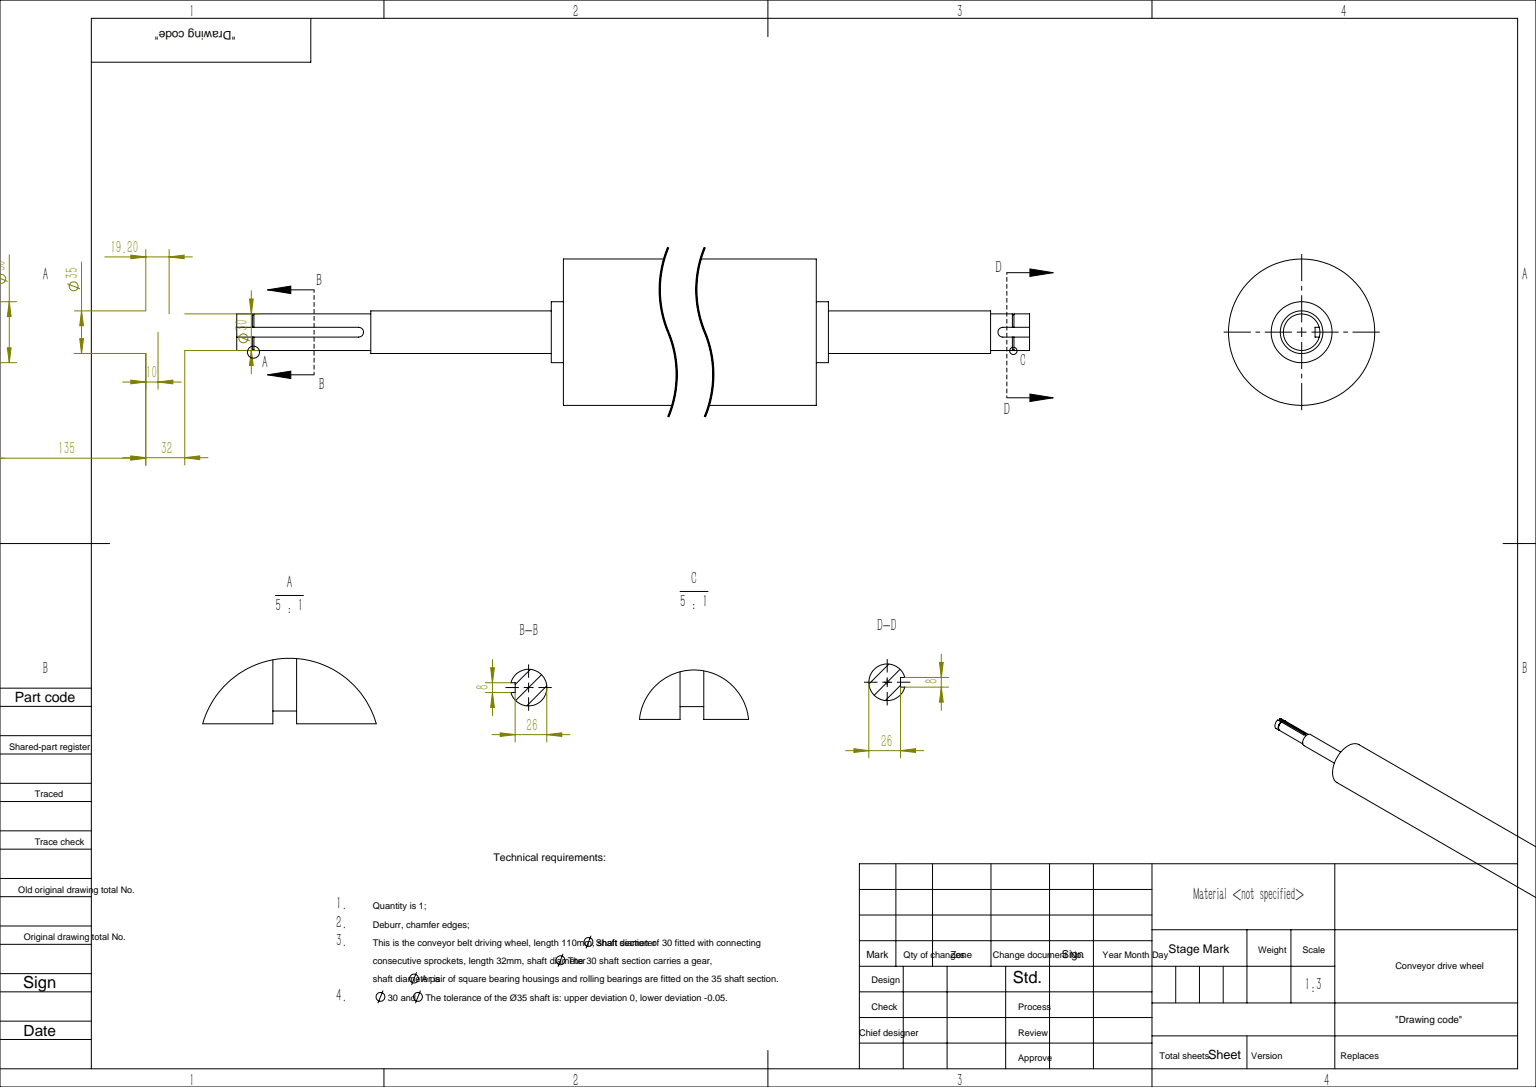
from build123d import *

# Parameters (mm, degrees)
CUT_EXTRUDE_1_DEPTH = 4
CUT_EXTRUDE_START   = -1.3
SKETCH_3_R          = 15
SKETCH_3_R_2        = 14.3
CUT_EXTRUDE_2_DEPTH = 1.3
CUT_EXTRUDE_3_DEPTH = 4
SKETCH_5_R          = 15
SKETCH_5_R_2        = 14.3
CUT_EXTRUDE_4_DEPTH = 1.3


with BuildPart() as part:
    # 草图1 → 旋转1 (revolve)
    with BuildSketch(Plane.XY, mode=Mode.PRIVATE) as revolve_1_sk:
        Polygon((0, 0), (0, 15), (110, 15), (110, 17.5), (258, 17.5), (258, 25), (268, 25), (268, 60), (1118, 60), (1118, 25), (1128, 25), (1128, 17.5), (1261, 17.5), (1261, 15), (1293, 15), (1293, 0), align=None)
    revolve(revolve_1_sk.sketch.rotate(Axis((0, 0, 0), (1, 0, 0)), 90), axis=Axis((0, 0, 0), (1, 0, 0)))

    # 草图2 → 切除-拉伸1 (cut)
    with BuildSketch(Plane(origin=(0, 15, 0), x_dir=(1, 0, 0), z_dir=(0, 1, 0))):
        with BuildLine():
            Line((100, 4), (-10, 4))
            Line((-10, 4), (-10, -4))
            Line((-10, -4), (100, -4))
            ThreePointArc((100, -4), (104, 0), (100, 4))
        make_face()
    extrude(amount=-CUT_EXTRUDE_1_DEPTH, mode=Mode.SUBTRACT)

    # 草图3 → 切除-拉伸2 (cut)
    with BuildSketch(Plane.ZY.offset(-12.8).offset(CUT_EXTRUDE_START)):
        Circle(SKETCH_3_R)
        Circle(SKETCH_3_R_2, mode=Mode.SUBTRACT)
    extrude(amount=CUT_EXTRUDE_2_DEPTH, mode=Mode.SUBTRACT)

    # 草图4 → 切除-拉伸3 (cut)
    with BuildSketch(Plane(origin=(0, 15, 0), x_dir=(1, 0, 0), z_dir=(0, 1, 0))):
        with BuildLine():
            Line((1271, 4), (1303, 4))
            Line((1303, 4), (1303, -4))
            Line((1303, -4), (1271, -4))
            ThreePointArc((1271, -4), (1267, 0), (1271, 4))
        make_face()
    extrude(amount=-CUT_EXTRUDE_3_DEPTH, mode=Mode.SUBTRACT)

    # 草图5 → 切除-拉伸4 (cut)
    with BuildSketch(Plane(origin=(1280.2, 0, 0), x_dir=(0, 0, -1), z_dir=(1, 0, 0))):
        with Locations(Location((0, 0, 0), (0, 0, 180))):
            Circle(SKETCH_5_R)
        Circle(SKETCH_5_R_2, mode=Mode.SUBTRACT)
    extrude(amount=-CUT_EXTRUDE_4_DEPTH, mode=Mode.SUBTRACT)


solid = part.part
